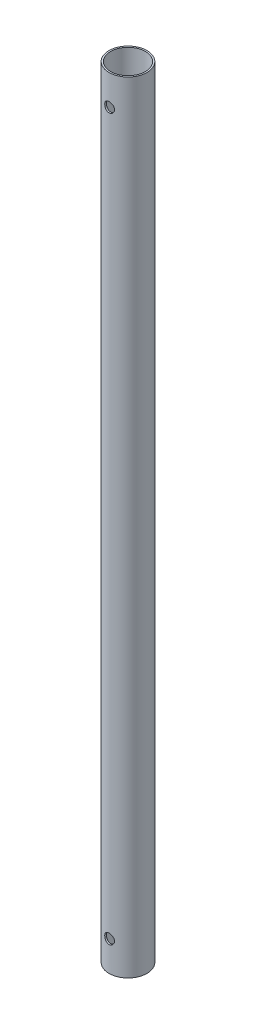
SolidWorks part; units mm, degrees
material "Thornel Mat VMA"
ref_plane "前视基准面" through (0, 0, 0) normal (0, 0, 1) x (1, 0, 0)
ref_plane "上视基准面" through (0, 0, 0) normal (0, 1, 0) x (1, 0, 0)
ref_plane "右视基准面" through (0, 0, 0) normal (1, 0, 0) x (0, 0, -1)
other "Configuration Table"
sketch "草图1" plane through (0, 0, 0) normal (0, 1, 0) x (1, 0, 0)
  circle A0 centre (0, 0) radius 6
  circle A1 centre (0, 0) radius 5.5
  dimension "D1" = 0.5
  dimension "D2" = 12
extrude "凸台-拉伸1" add sketch "草图1" along normal blind 246.5
sketch "草图2" plane through (0, 0, 0) normal (0, 0, 1) x (1, 0, 0)
  line L0 (0, 0) -> (0, 231.3076) construction
  line L1 (6, 246.5) -> (-6, 246.5) construction
  circle A0 centre (0, 237) radius 1.55
  circle A1 centre (0, 9.5) radius 1.55
  dimension "D1" = 3.1
  dimension "D2" = 9.5
  dimension "D3" = 9.5
extrude "切除-拉伸1" cut sketch "草图2" against normal through all both and the other way through all
